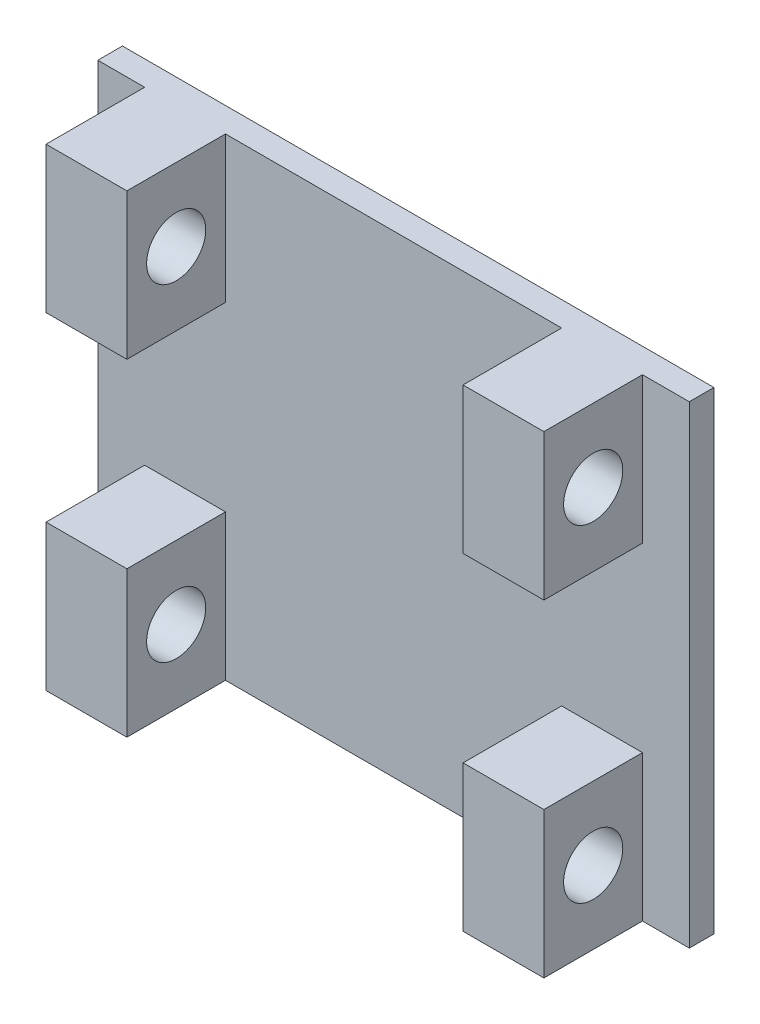
SolidWorks part; units mm, degrees
ref_plane "Front Plane" through (0, 0, 0) normal (0, 0, 1) x (1, 0, 0)
ref_plane "Top Plane" through (0, 0, 0) normal (0, 1, 0) x (1, 0, 0)
ref_plane "Right Plane" through (0, 0, 0) normal (1, 0, 0) x (0, 0, -1)
sketch "Sketch1" plane through (0, 0, 0) normal (0, 0, 1) x (1, 0, 0)
  line L0 (0, 0) -> (0, 480)
  line L1 (0, 480) -> (600, 480)
  line L2 (600, 480) -> (600, 0)
  line L3 (600, 0) -> (0, 0)
  dimension "D1" = 480
  dimension "D2" = 600
extrude "Boss-Extrude1" add sketch "Sketch1" along normal blind 25
sketch "Sketch2" plane through (0, 0, 25) normal (0, 0, 1) x (1, 0, 0)
  line L0 (47.5, 480) -> (47.5, 332)
  line L1 (552.5, 480) -> (552.5, 332)
  line L2 (47.5, 148) -> (129.5, 148)
  line L3 (47.5, 332) -> (129.5, 332)
  line L4 (0, 0) -> (600, 0)
  line L5 (600, 0) -> (600, 480)
  line L6 (600, 480) -> (0, 480)
  line L7 (0, 480) -> (0, 0)
  line L8 (47.5, 0) -> (129.5, 0)
  line L9 (600, 0) -> (600, 480) construction
  line L10 (552.5, 480) -> (47.5, 480)
  line L11 (0, 480) -> (0, 0) construction
  line L12 (129.5, 480) -> (129.5, 332)
  line L13 (470.5, 480) -> (470.5, 332)
  line L14 (47.5, 148) -> (47.5, 0)
  line L15 (47.5, 533.4972) -> (47.5, -52.4953) construction
  line L16 (129.5, 533.4972) -> (129.5, -52.4953) construction
  line L17 (129.5, 148) -> (129.5, 0)
  line L18 (470.5, 148) -> (552.5, 148)
  line L19 (470.5, 0) -> (552.5, 0)
  line L20 (470.5, 533.4972) -> (470.5, -102.9823) construction
  line L21 (552.5, 148) -> (552.5, 0)
  line L22 (552.5, 533.4972) -> (552.5, -102.9823) construction
  line L23 (470.5, 148) -> (470.5, 0)
  line L24 (470.5, 332) -> (600, 332)
  line M5 (0, 0) -> (600, 0)
  line M7 (600, 480) -> (0, 480)
  dimension "D2" = 47.5
  dimension "D3" = 47.5
  dimension "D4" = 148
  dimension "D5" = 148
  dimension "D1" = 0
  dimension "D6" = 82
  dimension "D7" = 82
extrude "Boss-Extrude2" add sketch "Sketch2" along normal blind 100 contours L12 L10 L0 L3 | L17 L2 L14 M5 | L18 L23 L21 M5 | L13 L24 L1 M7
sketch "Sketch4" plane through (47.5, 0, 0) normal (-1, 0, 0) x (0, 0, 1)
  line L0 (-159.2408, 74) -> (185.3189, 74) construction
  line L1 (125, 0) -> (25, 0) construction
  line L2 (75, 560.4514) -> (75, -122.719) construction
  line L3 (25, 480) -> (25, 0) construction
  line L4 (-136.0103, 406) -> (300.7933, 406) construction
  line L5 (125, 480) -> (25, 480) construction
  circle A0 centre (75, 406) radius 30
  circle A1 centre (75, 74) radius 30
  dimension "D4" = 60
  dimension "D5" = 60
  dimension "D1" = 74
  dimension "D2" = 50
  dimension "D3" = 74
extrude "Cut-Extrude1" cut sketch "Sketch4" against normal through all
sketch "Sketch5" plane through (0, 0, 0) normal (0, 0, -1) x (-1, 0, 0)
  line L0 (0, 480) -> (0, 0) construction
  line L1 (0, 480) -> (0, 0) construction
  line L2 (0, 0) -> (-600, 0) construction
  line L3 (0, 0) -> (-600, 0) construction
  line L4 (0, 240) -> (-880.1919, 240) construction
  line L5 (-300, 0) -> (-300, 656.8483) construction
  circle A0 centre (-300, 240) radius 65
  circle A1 centre (-300, 240) radius 40
  dimension "D1" = 130
  dimension "D2" = 80
extrude "Boss-Extrude3" add sketch "Sketch5" along normal blind 20
sketch "Sketch6" plane through (0, 0, -20) normal (0, 0, -1) x (-1, 0, 0)
  circle A0 centre (-300, 240) radius 40 construction
  circle A1 centre (-300, 240) radius 40
  circle A2 centre (-300, 240) radius 60
  dimension "D1" = 120
extrude "Boss-Extrude4" add sketch "Sketch6" along normal blind 77
sketch "Sketch7" plane through (0, 0, 0) normal (0, 0, -1) x (-1, 0, 0)
  circle A0 centre (-300, 240) radius 40 construction
  circle A1 centre (-300, 240) radius 40
extrude "Boss-Extrude5" add sketch "Sketch7" along normal blind 12.5
